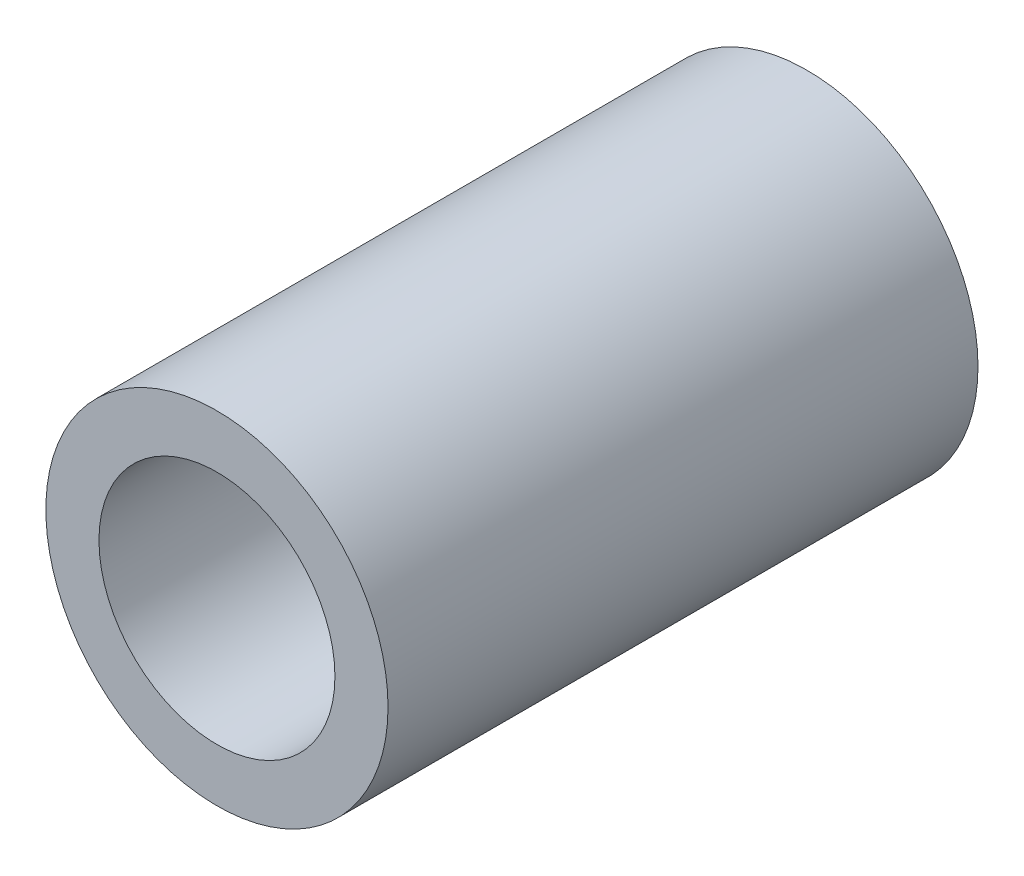
from build123d import *

# Parameters (mm, degrees)
SKETCH_1_R      = 14.5
SKETCH_1_R_2    = 10
EXTRUDE_1_DEPTH = 50


with BuildPart() as part:
    # 草图1 → 凸台-拉伸1 (new body)
    with BuildSketch(Plane.XY):
        Circle(SKETCH_1_R)
        Circle(SKETCH_1_R_2, mode=Mode.SUBTRACT)
    extrude(amount=EXTRUDE_1_DEPTH)


solid = part.part
